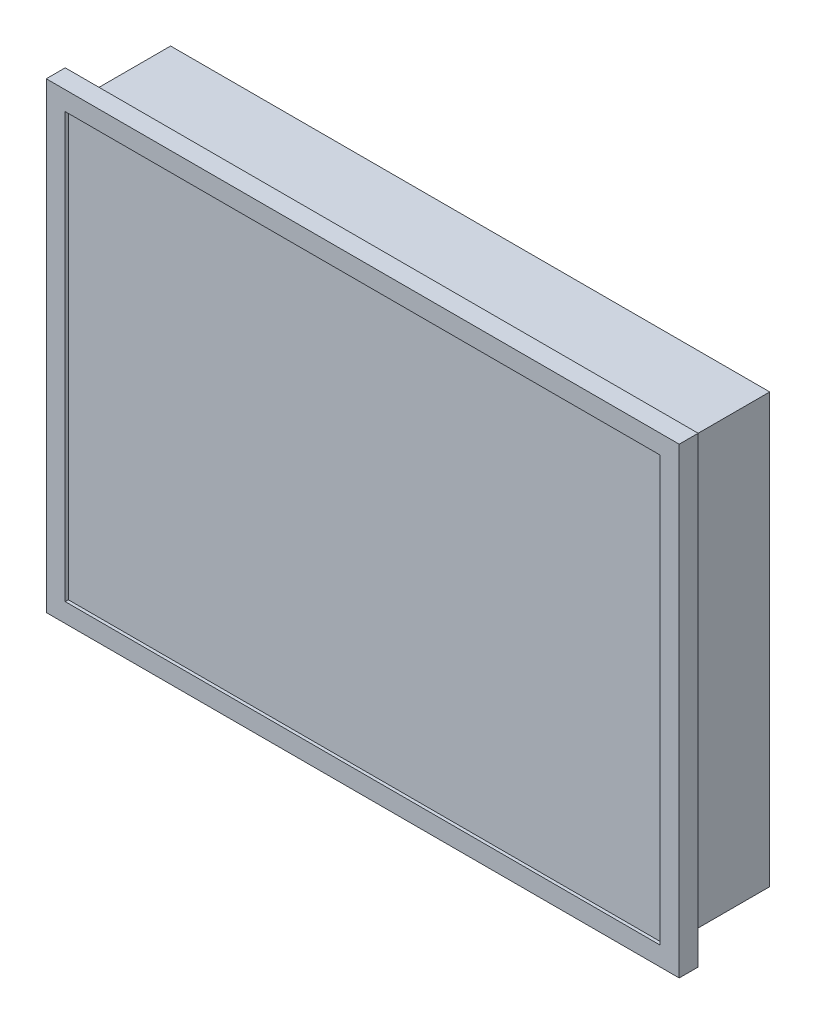
from build123d import *

# Parameters (mm, degrees)
SKETCH_1_W          = 200.3
SKETCH_1_H          = 146.3
EXTRUDE_1_DEPTH     = 6
SKETCH_2_W          = 189.6
SKETCH_2_H          = 135.6
EXTRUDE_2_DEPTH     = 28
SKETCH_3_W          = 188.3
SKETCH_3_H          = 134.3
CUT_EXTRUDE_1_DEPTH = 1


with BuildPart() as part:
    # 草图1 → 凸台-拉伸1 (new body)
    with BuildSketch(Plane.XY):
        Rectangle(SKETCH_1_W, SKETCH_1_H)
    extrude(amount=EXTRUDE_1_DEPTH)

    # 草图2 → 凸台-拉伸2 (add)
    with BuildSketch(Plane(origin=(0, 0, 0), x_dir=(-1, 0, 0), z_dir=(0, 0, -1))):
        Rectangle(SKETCH_2_W, SKETCH_2_H)
    extrude(amount=EXTRUDE_2_DEPTH)

    # 草图3 → 切除-拉伸1 (cut)
    with BuildSketch(Plane.XY.offset(6)):
        Rectangle(SKETCH_3_W, SKETCH_3_H)
    extrude(amount=-CUT_EXTRUDE_1_DEPTH, mode=Mode.SUBTRACT)


solid = part.part
